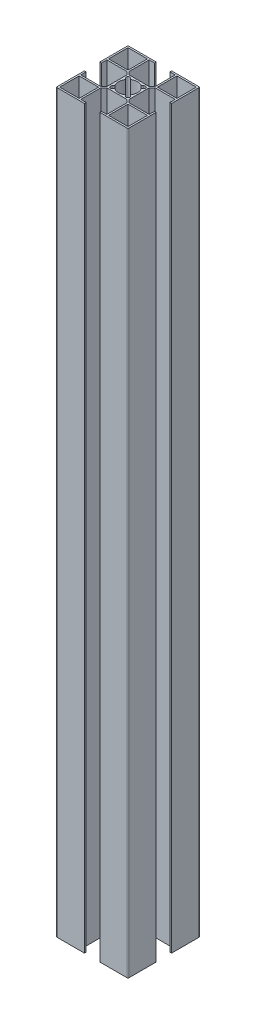
from build123d import *

# Parameters (mm, degrees)
SKETCH1_W               = 10.85
SKETCH1_H               = 10.85
BOSS_EXTRUDE1_DEPTH     = 410
MIRROR2_COPY_1_SKETCH_W = 10.85
MIRROR2_COPY_1_SKETCH_H = 10.85
MIRROR2_COPY_1_DEPTH    = 410


with BuildPart() as part:
    # Sketch1 → Boss-Extrude1 (new body)
    with BuildSketch(Plane(origin=(0, 0, 0), x_dir=(1, 0, 0), z_dir=(0, 1, 0))):
        with BuildLine():
            Line((-4.3, 20), (-19.5, 20))
            ThreePointArc((-19.5, 20), (-19.853553391, 19.853553391), (-20, 19.5))
            Line((-20, 19.5), (-20, 4.3))
            Line((-20, 4.3), (-19.05, 4.3))
            Line((-19.05, 4.3), (-19.05, 7.25))
            Line((-19.05, 7.25), (-7.921751442, 7.25))
            Line((-7.921751442, 7.25), (-6.2, 5.528248558))
            Line((-6.2, 5.528248558), (-6.2, 0))
            Line((-6.2, 0), (-5.3, 0))
            ThreePointArc((-5.3, 0), (-5.066731596, 1.555066215), (-4.387460025, 2.973246463))
            Line((-4.387460025, 2.973246463), (-5.091168825, 3.676955262))
            ThreePointArc((-5.091168825, 3.676955262), (-5.091168825, 5.091168825), (-3.676955262, 5.091168825))
            Line((-3.676955262, 5.091168825), (-2.973246463, 4.387460025))
            ThreePointArc((-2.973246463, 4.387460025), (-1.555066215, 5.066731596), (0, 5.3))
            Line((0, 5.3), (0, 6.2))
            Line((0, 6.2), (-5.528248558, 6.2))
            Line((-5.528248558, 6.2), (-7.25, 7.921751442))
            Line((-7.25, 7.921751442), (-7.25, 19.05))
            Line((-7.25, 19.05), (-4.3, 19.05))
            Line((-4.3, 19.05), (-4.3, 20))
        make_face()
        with Locations((-13.625, 13.625)):
            Rectangle(SKETCH1_W, SKETCH1_H, mode=Mode.SUBTRACT)
    boss_extrude1 = extrude(amount=BOSS_EXTRUDE1_DEPTH)

    # Mirror1: Boss-Extrude1 across plane
    add(boss_extrude1.mirror(Plane(origin=(0, 0, 0), x_dir=(0, 0, 1), z_dir=(1, 0, 0))))

    # Mirror2: Boss-Extrude1 across plane
    add(boss_extrude1.mirror(Plane.XY))

    # Mirror2 copy 1 sketch → Mirror2 copy 1 (add)
    with BuildSketch(Plane(origin=(0, 0, 0), x_dir=(-1, 0, 0), z_dir=(0, 1, 0))):
        with BuildLine():
            Line((-4.3, 20), (-19.5, 20))
            ThreePointArc((-19.5, 20), (-19.853553391, 19.853553391), (-20, 19.5))
            Line((-20, 19.5), (-20, 4.3))
            Line((-20, 4.3), (-19.05, 4.3))
            Line((-19.05, 4.3), (-19.05, 7.25))
            Line((-19.05, 7.25), (-7.921751442, 7.25))
            Line((-7.921751442, 7.25), (-6.2, 5.528248558))
            Line((-6.2, 5.528248558), (-6.2, 0))
            Line((-6.2, 0), (-5.3, 0))
            ThreePointArc((-5.3, 0), (-5.066731596, 1.555066215), (-4.387460025, 2.973246463))
            Line((-4.387460025, 2.973246463), (-5.091168825, 3.676955262))
            ThreePointArc((-5.091168825, 3.676955262), (-5.091168825, 5.091168825), (-3.676955262, 5.091168825))
            Line((-3.676955262, 5.091168825), (-2.973246463, 4.387460025))
            ThreePointArc((-2.973246463, 4.387460025), (-1.555066215, 5.066731596), (0, 5.3))
            Line((0, 5.3), (0, 6.2))
            Line((0, 6.2), (-5.528248558, 6.2))
            Line((-5.528248558, 6.2), (-7.25, 7.921751442))
            Line((-7.25, 7.921751442), (-7.25, 19.05))
            Line((-7.25, 19.05), (-4.3, 19.05))
            Line((-4.3, 19.05), (-4.3, 20))
        make_face()
        with Locations((-13.625, 13.625)):
            Rectangle(MIRROR2_COPY_1_SKETCH_W, MIRROR2_COPY_1_SKETCH_H, mode=Mode.SUBTRACT)
    extrude(amount=MIRROR2_COPY_1_DEPTH)


solid = part.part
